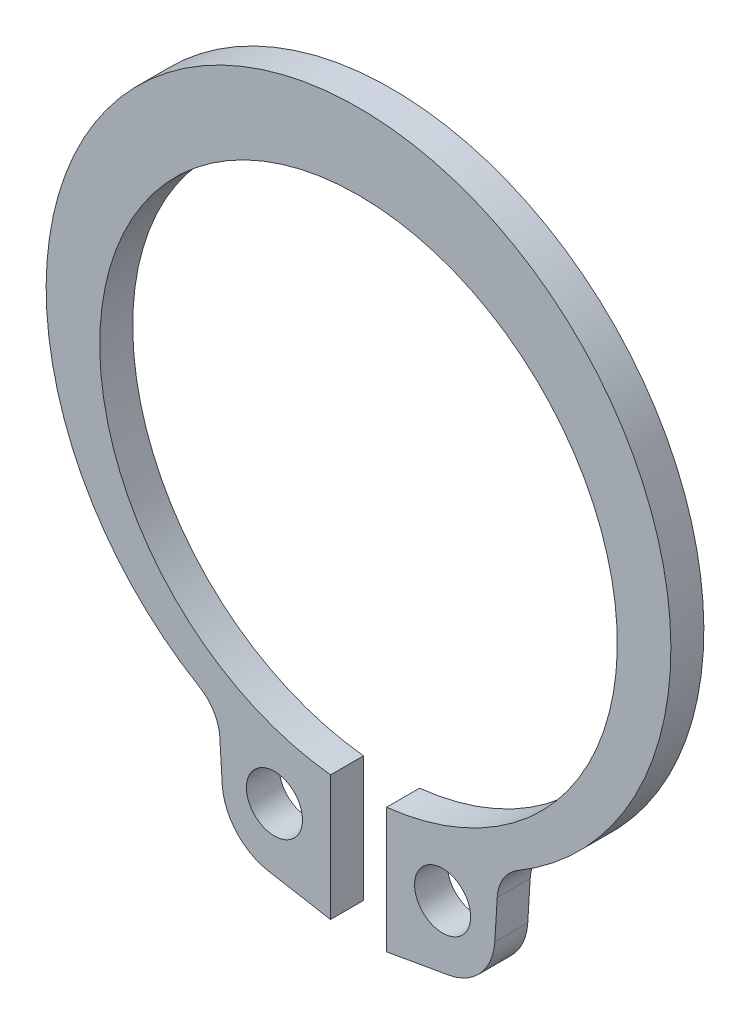
from build123d import *

# Parameters (mm, degrees)
SKETCH_2_R      = 0.85
EXTRUDE_1_DEPTH = 0.5
FILLET_1_R      = 1.266666667


with BuildPart() as part:
    # 草图2 → 凸台-拉伸1 (new, symmetric)
    with BuildSketch(Plane.XY):
        with BuildLine():
            Line((4.133871572, -9.701079585), (4.25, -7.793360231))
            ThreePointArc((4.25, -7.793360231), (0, 10.15), (-4.25, -7.793360231))
            Line((-4.25, -7.793360231), (-4.133871572, -9.701079585))
            ThreePointArc((-4.133871572, -9.701079585), (-3.705473422, -10.72960262), (-2.732214432, -11.271960018))
            Line((-2.732214432, -11.271960018), (-0.85, -11.603845206))
            Line((-0.85, -11.603845206), (-0.85, -7.803845206))
            ThreePointArc((-0.85, -7.803845206), (0, 7.85), (0.85, -7.803845206))
            Line((0.85, -7.803845206), (0.85, -11.603845206))
            Line((0.85, -11.603845206), (2.732214432, -11.271960018))
            ThreePointArc((2.732214432, -11.271960018), (3.705473422, -10.72960262), (4.133871572, -9.701079585))
        make_face()
        with Locations((2.55, -9.410632285)):
            Circle(SKETCH_2_R, mode=Mode.SUBTRACT)
        with Locations(Location((-2.55, -9.410632285, 0), (0, 0, 180))):
            Circle(SKETCH_2_R, mode=Mode.SUBTRACT)
    extrude(amount=EXTRUDE_1_DEPTH, both=True)

    # 圆角1
    fillet_1_edges = [part.edges().sort_by_distance(p)[0] for p in [
        (-4.25, -7.793360231, 0),
        (4.25, -7.793360231, 0),
    ]]
    fillet(fillet_1_edges, radius=FILLET_1_R)


solid = part.part
